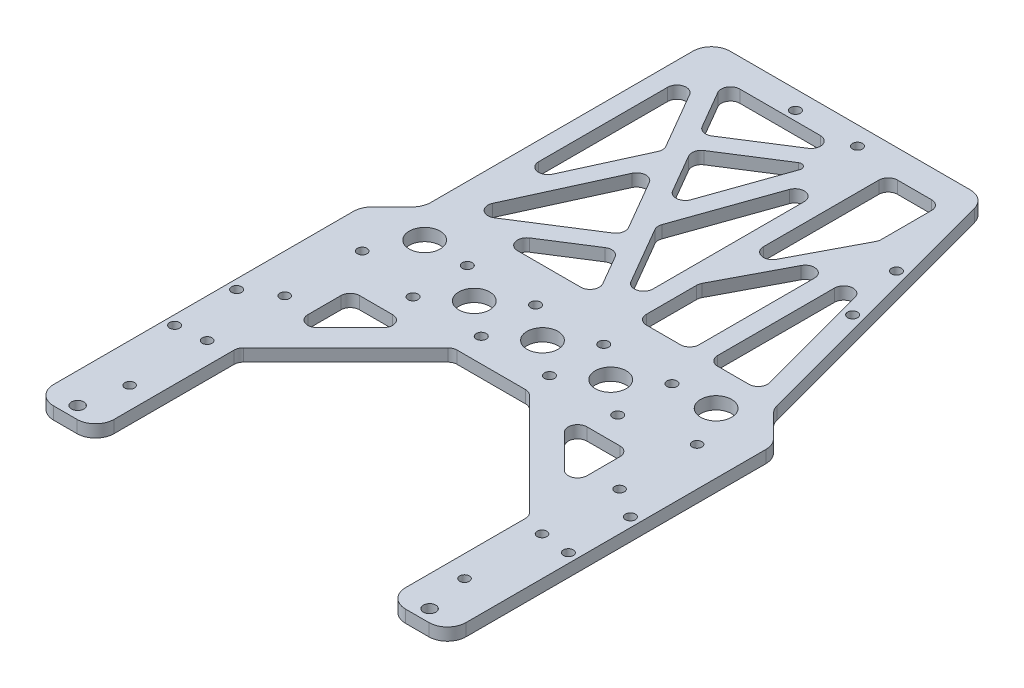
from build123d import *
from OCP.BRepFilletAPI import BRepFilletAPI_MakeFillet

# Parameters (mm, degrees)
SKETCH_1_R          = 1.55
EXTRUDE_1_DEPTH     = 4
CUT_EXTRUDE_1_DEPTH = 139.25907746
CUT_EXTRUDE_2_DEPTH = 420
FILLET_1_R          = 3
SKETCH_4_R          = 1.6
CUT_EXTRUDE_3_DEPTH = 139.25907746
SKETCH_5_R          = 1.6
CUT_EXTRUDE_4_DEPTH = 10
CHAMFER_1_SIZE      = 10
EXTRUDE_2_DEPTH     = 4
SKETCH_8_R          = 1.6
CUT_EXTRUDE_6_DEPTH = 4
FILLET_2_R          = 6
SKETCH_7_R          = 5
CUT_EXTRUDE_5_DEPTH = 4
FILLET_3_R1         = 3
FILLET_3_R2         = 1.5
SKETCH_9_R          = 2
SKETCH_9_W          = 133
SKETCH_9_H          = 6
CUT_EXTRUDE_7_DEPTH = 10
FILLET_4_R          = 6


with BuildPart() as part:
    # 草图1 → 凸台-拉伸1 (new body)
    with BuildSketch(Plane(origin=(0, 0, 0), x_dir=(1, 0, 0), z_dir=(0, 1, 0))):
        Polygon((66.5, 0), (-66.5, 0), (-66.5, -121.15), (-41.5, -121.15), (-41.5, -71.5), (-10, -40), (10, -40), (41.5, -71.5), (41.5, -121.15), (66.5, -121.15), align=None)
        with Locations(Location((-54, -22.15, 0), (0, 0, 270))):
            Circle(SKETCH_1_R, mode=Mode.SUBTRACT)
        with Locations(Location((54, -22.15, 0), (0, 0, 270))):
            Circle(SKETCH_1_R, mode=Mode.SUBTRACT)
        with Locations(Location((-54, -47.15, 0), (0, 0, 270))):
            Circle(SKETCH_1_R, mode=Mode.SUBTRACT)
        with Locations(Location((54, -47.15, 0), (0, 0, 270))):
            Circle(SKETCH_1_R, mode=Mode.SUBTRACT)
        with Locations(Location((-54, -72.15, 0), (0, 0, 270))):
            Circle(SKETCH_1_R, mode=Mode.SUBTRACT)
        with Locations(Location((54, -72.15, 0), (0, 0, 270))):
            Circle(SKETCH_1_R, mode=Mode.SUBTRACT)
        with Locations(Location((-54, -97.15, 0), (0, 0, 270))):
            Circle(SKETCH_1_R, mode=Mode.SUBTRACT)
        with Locations(Location((54, -97.15, 0), (0, 0, 270))):
            Circle(SKETCH_1_R, mode=Mode.SUBTRACT)
    extrude(amount=EXTRUDE_1_DEPTH)

    # 草图2 → 切除-拉伸1 (cut, through all)
    with BuildSketch(Plane(origin=(0, 4, 0), x_dir=(1, 0, 0), z_dir=(0, 1, 0))):
        Polygon((-47, -115.65), (-47, -121.15), (47, -121.15), (47, -115.65), (47, -69.221825407), (12.278174593, -34.5), (-12.278174593, -34.5), (-47, -69.221825407), align=None)
    extrude(amount=-CUT_EXTRUDE_1_DEPTH, mode=Mode.SUBTRACT)

    # 草图3 → 切除-拉伸2 (cut)
    with BuildSketch(Plane(origin=(0, 4, 0), x_dir=(1, 0, 0), z_dir=(0, 1, 0))):
        Polygon((-45, -55.908116908), (-45, -35), (-24.091883092, -35), align=None)
        Polygon((24.091883092, -35), (45, -55.908116908), (45, -35), align=None)
    extrude(amount=-CUT_EXTRUDE_2_DEPTH, mode=Mode.SUBTRACT)

    # 圆角1
    fillet_1_edges = [part.edges().sort_by_distance(p)[0] for p in [
        (-24.091883092, 2, 35),
        (-45, 2, 55.908116908),
        (-45, 2, 35),
        (24.091883092, 2, 35),
        (45, 2, 35),
        (45, 2, 55.908116908),
        (-47, 2, 69.221825407),
        (-12.278174593, 2, 34.5),
        (12.278174593, 2, 34.5),
        (47, 2, 69.221825407),
    ]]
    fillet(fillet_1_edges, radius=FILLET_1_R)

    # 草图4 → 切除-拉伸3 (cut, through all)
    with BuildSketch(Plane(origin=(0, 4, 0), x_dir=(1, 0, 0), z_dir=(0, 1, 0))):
        with Locations(Location((-33, -26.75, 0), (0, 0, 270))):
            Circle(SKETCH_4_R)
        with Locations(Location((33, -26.75, 0), (0, 0, 270))):
            Circle(SKETCH_4_R)
        with Locations(Location((-33, -9.25, 0), (0, 0, 270))):
            Circle(SKETCH_4_R)
        with Locations(Location((11, -9.25, 0), (0, 0, 270))):
            Circle(SKETCH_4_R)
        with Locations(Location((-11, -9.25, 0), (0, 0, 270))):
            Circle(SKETCH_4_R)
        with Locations(Location((33, -9.25, 0), (0, 0, 270))):
            Circle(SKETCH_4_R)
        with Locations(Location((11, -26.75, 0), (0, 0, 270))):
            Circle(SKETCH_4_R)
        with Locations(Location((-11, -26.75, 0), (0, 0, 270))):
            Circle(SKETCH_4_R)
    extrude(amount=-CUT_EXTRUDE_3_DEPTH, mode=Mode.SUBTRACT)

    # 草图5 → 切除-拉伸4 (cut)
    with BuildSketch(Plane(origin=(0, 4, 0), x_dir=(1, 0, 0), z_dir=(0, 1, 0))):
        with Locations(Location((-63.5, -53.15, 0), (0, 0, 270))):
            Circle(SKETCH_5_R)
        with Locations(Location((63.5, -53.15, 0), (0, 0, 270))):
            Circle(SKETCH_5_R)
        with Locations(Location((-63.5, -73.15, 0), (0, 0, 270))):
            Circle(SKETCH_5_R)
        with Locations(Location((63.5, -73.15, 0), (0, 0, 270))):
            Circle(SKETCH_5_R)
    extrude(amount=-CUT_EXTRUDE_4_DEPTH, mode=Mode.SUBTRACT)

    # 倒角1
    chamfer_1_edges = [part.edges().sort_by_distance(p)[0] for p in [
        (-66.5, 2, 0),
        (66.5, 2, 0),
    ]]
    chamfer(chamfer_1_edges, length=CHAMFER_1_SIZE)

    # 草图6 → 凸台-拉伸2 (add)
    with BuildSketch(Plane(origin=(0, 4, 0), x_dir=(1, 0, 0), z_dir=(0, 1, 0))):
        Polygon((-56.5, 93), (-56.5, 0), (56.5, 0), (31.580725104, 93), align=None)
    extrude(amount=-EXTRUDE_2_DEPTH)

    # 草图8 → 切除-拉伸6 (cut)
    with BuildSketch(Plane(origin=(0, 4, 0), x_dir=(1, 0, 0), z_dir=(0, 1, 0))):
        with Locations(Location((-23.419274896, 87, 0), (0, 0, 270))):
            Circle(SKETCH_8_R)
        with Locations(Location((-3.419274896, 87, 0), (0, 0, 270))):
            Circle(SKETCH_8_R)
        with Locations(Location((37.741614204, 58.416138945, 0), (0, 0, 270))):
            Circle(SKETCH_8_R)
        with Locations(Location((42.917995106, 39.097622419, 0), (0, 0, 270))):
            Circle(SKETCH_8_R)
    extrude(amount=-CUT_EXTRUDE_6_DEPTH, mode=Mode.SUBTRACT)

    # 圆角2
    fillet_2_edges = [part.edges().sort_by_distance(p)[0] for p in [
        (66.5, 2, 121.15),
        (-66.5, 2, 121.15),
        (-56.5, 2, 0),
        (56.5, 2, 0),
        (66.5, 2, 10),
        (-66.5, 2, 10),
        (-56.5, 2, -93),
        (31.580725104, 2, -93),
        (47, 2, 121.15),
        (-47, 2, 121.15),
    ]]
    fillet(fillet_2_edges, radius=FILLET_2_R)

    # 草图7 → 切除-拉伸5 (cut)
    with BuildSketch(Plane(origin=(0, 4, 0), x_dir=(1, 0, 0), z_dir=(0, 1, 0))):
        with Locations(Location((-22, -18, 0), (0, 0, 270))):
            Circle(SKETCH_7_R)
        with Locations(Location((0, -18, 0), (0, 0, 270))):
            Circle(SKETCH_7_R)
        with Locations(Location((22, -18, 0), (0, 0, 270))):
            Circle(SKETCH_7_R)
        with Locations(Location((47, -9, 0), (0, 0, 270))):
            Circle(SKETCH_7_R)
        with Locations(Location((-47, -9, 0), (0, 0, 90))):
            Circle(SKETCH_7_R)
        Polygon((-50.5, 84), (-50.5, 17.458578786), (-33.5, 54.730699229), align=None)
        Polygon((-39.333035497, 3), (-3.454120401, 3), (-13.144398267, 19.683979847), align=None)
        Polygon((-43.561384259, 84), (-2.098986911, 84), (-32.36310387, 64.719656659), align=None)
        Polygon((-4.723403201, 75.213933081), (-17.473403201, 39.083707996), (-29.347098825, 59.52692967), align=None)
        Polygon((-13.51550466, 32.269300771), (3.48449534, 80.442934218), (3.48449534, 3), align=None)
        Polygon((9.48449534, 84), (9.48449534, 31.60760773), (26.48449534, 64), (26.48449534, 84), align=None)
        Polygon((32.48449534, 66.444863729), (49.48449534, 3), (32.48449534, 3), align=None)
        Polygon((26.48449534, 55.39239227), (9.48449534, 23), (9.48449534, 3), (26.48449534, 3), align=None)
        Polygon((-29.80612279, 48.370863754), (-50.5, 3), (-16.160403312, 24.876706835), align=None)
    extrude(amount=-CUT_EXTRUDE_5_DEPTH, mode=Mode.SUBTRACT)

    # 圆角3: one fillet with a radius per group of edges: ONE call of the kernel's fillet builder (fillet() takes one radius for all edges)
    fillet_3_edges_1 = [part.edges().sort_by_distance(p)[0] for p in [
        (26.48449534, 2, -84),
        (9.48449534, 2, -84),
        (9.48449534, 2, -31.60760773),
        (26.48449534, 2, -64),
        (-13.51550466, 2, -32.269300771),
        (3.48449534, 2, -3),
        (3.48449534, 2, -80.442934218),
        (-17.473403201, 2, -39.083707996),
        (-3.454120401, 2, -3),
        (32.48449534, 2, -66.444863729),
        (32.48449534, 2, -3),
        (49.48449534, 2, -3),
        (26.48449534, 2, -3),
        (26.48449534, 2, -55.39239227),
        (9.48449534, 2, -23),
        (9.48449534, 2, -3),
        (-33.5, 2, -54.730699229),
        (-50.5, 2, -84),
        (-50.5, 2, -17.458578786),
        (-43.561384259, 2, -84),
        (-29.347098825, 2, -59.52692967),
        (-13.144398267, 2, -19.683979847),
        (-39.333035497, 2, -3),
        (-32.36310387, 2, -64.719656659),
        (-2.098986911, 2, -84),
        (-16.160403312, 2, -24.876706835),
        (-29.80612279, 2, -48.370863754),
        (-50.5, 2, -3),
    ]]
    fillet_3_edges_2 = [part.edges().sort_by_distance(p)[0] for p in [
        (-4.723403201, 2, -75.213933081),
    ]]
    fillet_3 = BRepFilletAPI_MakeFillet(part.part.solid().wrapped)
    for e in fillet_3_edges_1:
        fillet_3.Add(FILLET_3_R1, e.wrapped)
    for e in fillet_3_edges_2:
        fillet_3.Add(FILLET_3_R2, e.wrapped)
    add(Compound.cast(fillet_3.Shape()), mode=Mode.REPLACE)

    # 草图9 → 切除-拉伸7 (cut)
    with BuildSketch(Plane(origin=(0, 4, 0), x_dir=(1, 0, 0), z_dir=(0, 1, 0))):
        with Locations(Location((-56.75, -111.15, 0), (0, 0, 270))):
            Circle(SKETCH_9_R)
        with Locations(Location((56.75, -111.15, 0), (0, 0, 270))):
            Circle(SKETCH_9_R)
        with Locations((0, -118.15)):
            Rectangle(SKETCH_9_W, SKETCH_9_H)
    extrude(amount=-CUT_EXTRUDE_7_DEPTH, mode=Mode.SUBTRACT)

    # 圆角4
    fillet_4_edges = [part.edges().sort_by_distance(p)[0] for p in [
        (66.5, 2, 115.15),
        (47, 2, 115.15),
        (-47, 2, 115.15),
        (-66.5, 2, 115.15),
    ]]
    fillet(fillet_4_edges, radius=FILLET_4_R)


solid = part.part
